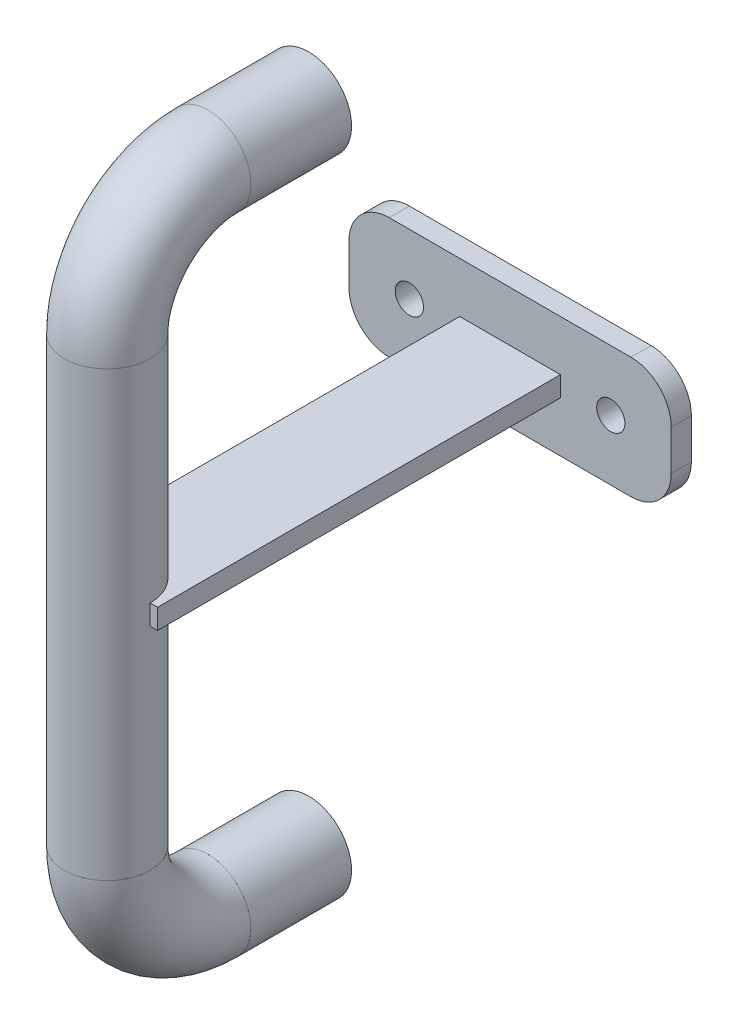
from build123d import *

# Parameters (mm, degrees)
SKETCH_1_W                                    = 80
SKETCH_1_H                                    = 30
SKETCH_1_R                                    = 3.5
SKETCH_1_W_2                                  = 25
SKETCH_1_H_2                                  = 5
BOSS_EXTRUDE1_DEPTH                           = 5
FILLET1_R                                     = 10
SKETCH4_W                                     = 25
SKETCH4_H                                     = 5
BOSS_EXTRUDE2_DEPTH                           = 100
SKETCH5_R                                     = 10.5
CUT_EXTRUDE1_DEPTH                            = 134.158739856
SKETCH1_R                                     = 10.65
SKETCH1_R_2                                   = 9.45
GB_T_6728_2002_ROUND_TUBE_021_3_X_1_2_2_DEPTH = 110
SKETCH1_ON_SEGMENT_2_R                        = 10.65
SKETCH1_ON_SEGMENT_2_R_2                      = 9.45
GB_T_6728_2002_ROUND_TUBE_021_3_X_1_2_ANGLE   = 90
SKETCH1_ON_SEGMENT_3_R                        = 10.65
SKETCH1_ON_SEGMENT_3_R_2                      = 9.45
GB_T_6728_2002_ROUND_TUBE_021_3_X_1_3_ANGLE   = 90
SKETCH1_ON_SEGMENT_4_R                        = 10.65
SKETCH1_ON_SEGMENT_4_R_2                      = 9.45
GB_T_6728_2002_ROUND_TUBE_021_3_X_1_4_DEPTH   = 25
SKETCH1_ON_SEGMENT_5_R                        = 10.65
SKETCH1_ON_SEGMENT_5_R_2                      = 9.45
GB_T_6728_2002_ROUND_TUBE_021_3_X_1_5_DEPTH   = 25


with BuildPart() as part:
    # Sketch 1 → Boss-Extrude1 (new body)
    with BuildSketch(Plane.XY):
        with Locations((40, -15)):
            Rectangle(SKETCH_1_W, SKETCH_1_H)
        with Locations((15, -15)):
            Circle(SKETCH_1_R, mode=Mode.SUBTRACT)
        with Locations((65, -15)):
            Circle(SKETCH_1_R, mode=Mode.SUBTRACT)
        with Locations((40, -15)):
            Rectangle(SKETCH_1_W_2, SKETCH_1_H_2, mode=Mode.SUBTRACT)
    extrude(amount=BOSS_EXTRUDE1_DEPTH)

    # Fillet1
    fillet1_edges = [part.edges().sort_by_distance(p)[0] for p in [
        (0, 0, 2.5),
        (80, 0, 2.5),
        (80, -30, 2.5),
        (0, -30, 2.5),
    ]]
    fillet(fillet1_edges, radius=FILLET1_R)


with BuildPart() as body_2:
    # Sketch4 → Boss-Extrude2 (new body)
    with BuildSketch(Plane.XY.offset(5)):
        with Locations((40, -15)):
            Rectangle(SKETCH4_W, SKETCH4_H)
    extrude(amount=BOSS_EXTRUDE2_DEPTH)

    # Sketch5 → Cut-Extrude1 (cut, through all)
    with BuildSketch(Plane.XZ.offset(17.5)):
        with Locations((40, 105)):
            Circle(SKETCH5_R)
    extrude(amount=-CUT_EXTRUDE1_DEPTH, mode=Mode.SUBTRACT)


with BuildPart() as body_3:
    # Sketch1 → GB/T 6728-2002 round tube 021.3 X 1.2(2) (new body)
    with BuildSketch(Plane(origin=(40, 40, 105), x_dir=(1, 0, 0), z_dir=(0, -1, 0))):
        Circle(SKETCH1_R)
        Circle(SKETCH1_R_2, mode=Mode.SUBTRACT)
    extrude(amount=GB_T_6728_2002_ROUND_TUBE_021_3_X_1_2_2_DEPTH)


with BuildPart() as body_4:
    # Sketch1 on segment 2 (carried to the start of arc 2) → GB_T 6728-2002 round tube 021.3 X 1. 2 (revolve)
    with BuildSketch(Plane(origin=(40, 40, 105), x_dir=(1, 0, 0), z_dir=(0, 1, 0))):
        Circle(SKETCH1_ON_SEGMENT_2_R)
        Circle(SKETCH1_ON_SEGMENT_2_R_2, mode=Mode.SUBTRACT)
    revolve(axis=Axis((40, 40, 80), (-1, 0, 0)), revolution_arc=GB_T_6728_2002_ROUND_TUBE_021_3_X_1_2_ANGLE)


with BuildPart() as body_5:
    # Sketch1 on segment 3 (carried to the start of arc 3) → GB_T 6728-2002 round tube 021.3 X 1. 3 (revolve)
    with BuildSketch(Plane(origin=(40, -70, 105), x_dir=(1, 0, 0), z_dir=(0, -1, 0))):
        Circle(SKETCH1_ON_SEGMENT_3_R)
        Circle(SKETCH1_ON_SEGMENT_3_R_2, mode=Mode.SUBTRACT)
    revolve(axis=Axis((40, -70, 80), (1, 0, 0)), revolution_arc=GB_T_6728_2002_ROUND_TUBE_021_3_X_1_3_ANGLE)


with BuildPart() as body_6:
    # Sketch1 on segment 4 (carried to segment 4) → GB_T 6728-2002 round tube 021.3 X 1. 4 (new body)
    with BuildSketch(Plane(origin=(40, -95, 80), x_dir=(1, 0, 0), z_dir=(0, 0, -1))):
        Circle(SKETCH1_ON_SEGMENT_4_R)
        Circle(SKETCH1_ON_SEGMENT_4_R_2, mode=Mode.SUBTRACT)
    extrude(amount=GB_T_6728_2002_ROUND_TUBE_021_3_X_1_4_DEPTH)


with BuildPart() as body_7:
    # Sketch1 on segment 5 (carried to segment 5) → GB_T 6728-2002 round tube 021.3 X 1. 5 (new body)
    with BuildSketch(Plane(origin=(40, 65, 80), x_dir=(1, 0, 0), z_dir=(0, 0, -1))):
        Circle(SKETCH1_ON_SEGMENT_5_R)
        Circle(SKETCH1_ON_SEGMENT_5_R_2, mode=Mode.SUBTRACT)
    extrude(amount=GB_T_6728_2002_ROUND_TUBE_021_3_X_1_5_DEPTH)


solid = Compound([part.part, body_2.part, body_3.part, body_4.part, body_5.part, body_6.part, body_7.part])
